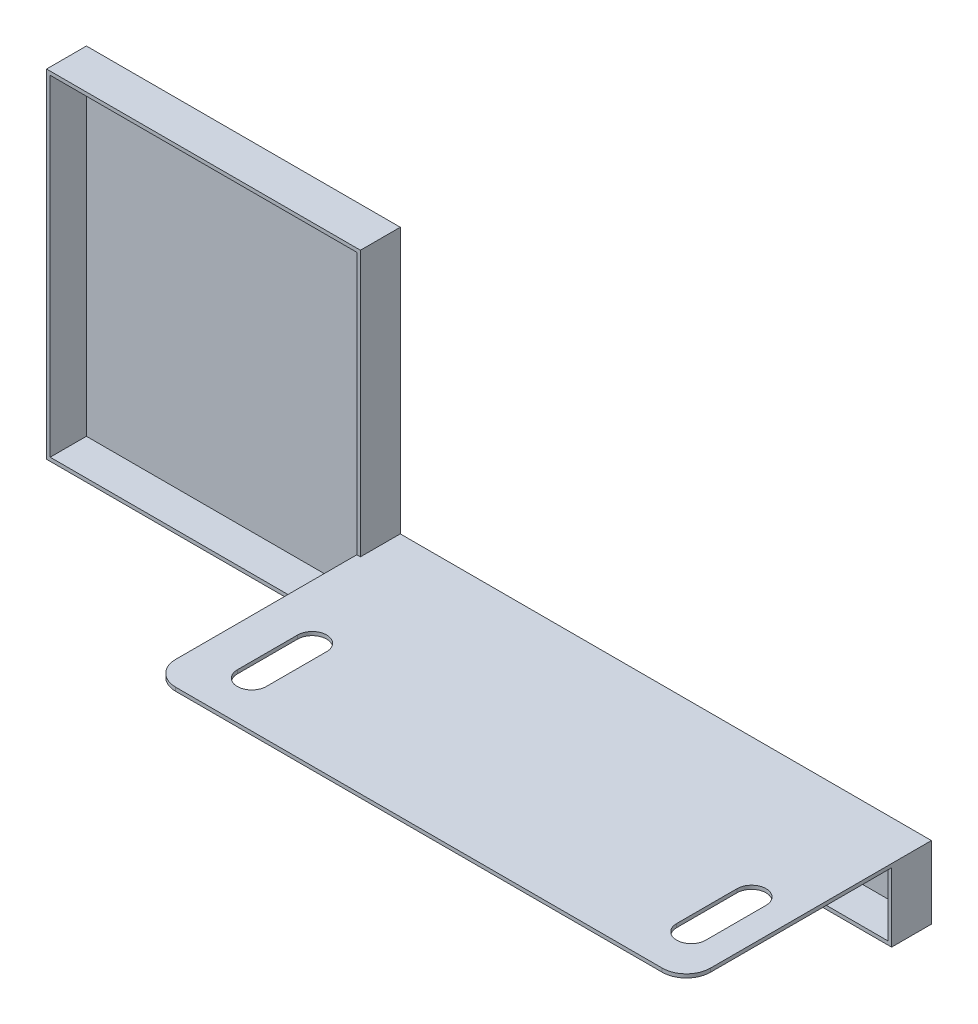
from build123d import *

# Parameters (mm, degrees)
SKETCH_1_W          = 350
SKETCH_1_H          = 140
EXTRUDE_1_DEPTH     = 1.5
SKETCH_2_W          = 220
SKETCH_2_H          = 110
CUT_EXTRUDE_1_DEPTH = 2
EXTRUDE_1_2_DEPTH   = 15
SKETCH_4_W          = 221.5
SKETCH_4_H          = 1.5
EXTRUDE_3_DEPTH     = 100
FILLET_1_R          = 10
CUT_EXTRUDE_2_DEPTH = 100


with BuildPart() as part:
    # 草图1 → Extrude 1 (new body)
    with BuildSketch(Plane.XY):
        Rectangle(SKETCH_1_W, SKETCH_1_H)
    extrude(amount=EXTRUDE_1_DEPTH)

    # 草图2 → 切除-拉伸1 (cut)
    with BuildSketch(Plane.XY.offset(1.5)):
        with Locations((65, 15)):
            Rectangle(SKETCH_2_W, SKETCH_2_H)
    extrude(amount=-CUT_EXTRUDE_1_DEPTH, mode=Mode.SUBTRACT)

    # 草图3 → Extrude 1 2 (add)
    with BuildSketch(Plane.XY.offset(1.5)):
        Polygon((175, -40), (175, -70), (-175, -70), (-175, 70), (-45, 70), (-45, -40), (-46.5, -40), (-46.5, 68.5), (-173.5, 68.5), (-173.5, -68.5), (173.5, -68.5), (173.5, -40), align=None)
    extrude(amount=EXTRUDE_1_2_DEPTH)

    # 草图4 → 凸台-拉伸3 (add)
    with BuildSketch(Plane.XY.offset(1.5)):
        with Locations((64.25, -40.75)):
            Rectangle(SKETCH_4_W, SKETCH_4_H)
    extrude(amount=EXTRUDE_3_DEPTH)

    # 圆角1
    fillet_1_edges = [part.edges().sort_by_distance(p)[0] for p in [
        (-46.5, -40.75, 101.5),
        (175, -40.75, 101.5),
    ]]
    fillet(fillet_1_edges, radius=FILLET_1_R)

    # 草图5 → 切除-拉伸2 (cut)
    with BuildSketch(Plane.XZ.offset(41.5)):
        with BuildLine():
            Line((-18, 82.5), (-18, 57.5))
            ThreePointArc((-18, 57.5), (-24, 51.5), (-30, 57.5))
            Line((-30, 57.5), (-30, 82.5))
            ThreePointArc((-30, 82.5), (-24, 88.5), (-18, 82.5))
        make_face()
        with BuildLine():
            Line((164, 82.5), (164, 57.5))
            ThreePointArc((164, 57.5), (158, 51.5), (152, 57.5))
            Line((152, 57.5), (152, 82.5))
            ThreePointArc((152, 82.5), (158, 88.5), (164, 82.5))
        make_face()
    extrude(amount=-CUT_EXTRUDE_2_DEPTH, mode=Mode.SUBTRACT)


solid = part.part
